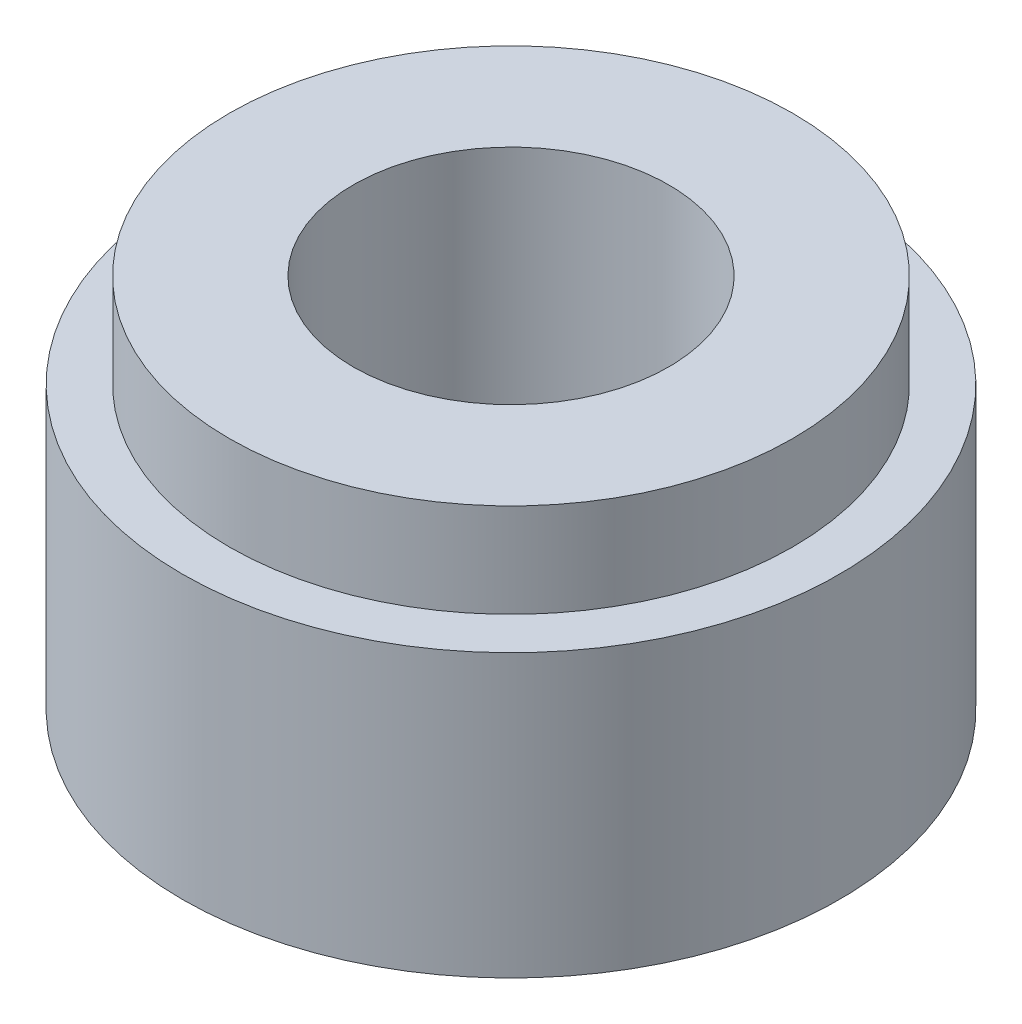
from build123d import *

# Parameters (mm, degrees)
SKETCH1_R           = 17.5
BOSS_EXTRUDE1_DEPTH = 15
SKETCH2_R           = 15
BOSS_EXTRUDE2_DEPTH = 5
SKETCH3_R           = 8.4
CUT_EXTRUDE1_DEPTH  = 32.819805153


with BuildPart() as part:
    # Sketch1 → Boss-Extrude1 (new body)
    with BuildSketch(Plane(origin=(0, 0, 0), x_dir=(1, 0, 0), z_dir=(0, 1, 0))):
        with Locations(Location((0, 0, 0), (0, 0, 270))):
            Circle(SKETCH1_R)
    extrude(amount=BOSS_EXTRUDE1_DEPTH)

    # Sketch2 → Boss-Extrude2 (add)
    with BuildSketch(Plane(origin=(0, 15, 0), x_dir=(1, 0, 0), z_dir=(0, 1, 0))):
        with Locations(Location((0, 0, 0), (0, 0, 270))):
            Circle(SKETCH2_R)
    extrude(amount=BOSS_EXTRUDE2_DEPTH)

    # Sketch3 → Cut-Extrude1 (cut, through all)
    with BuildSketch(Plane(origin=(0, 20, 0), x_dir=(1, 0, 0), z_dir=(0, 1, 0))):
        with Locations(Location((0, 0, 0), (0, 0, 270))):
            Circle(SKETCH3_R)
    extrude(amount=-CUT_EXTRUDE1_DEPTH, mode=Mode.SUBTRACT)


solid = part.part
